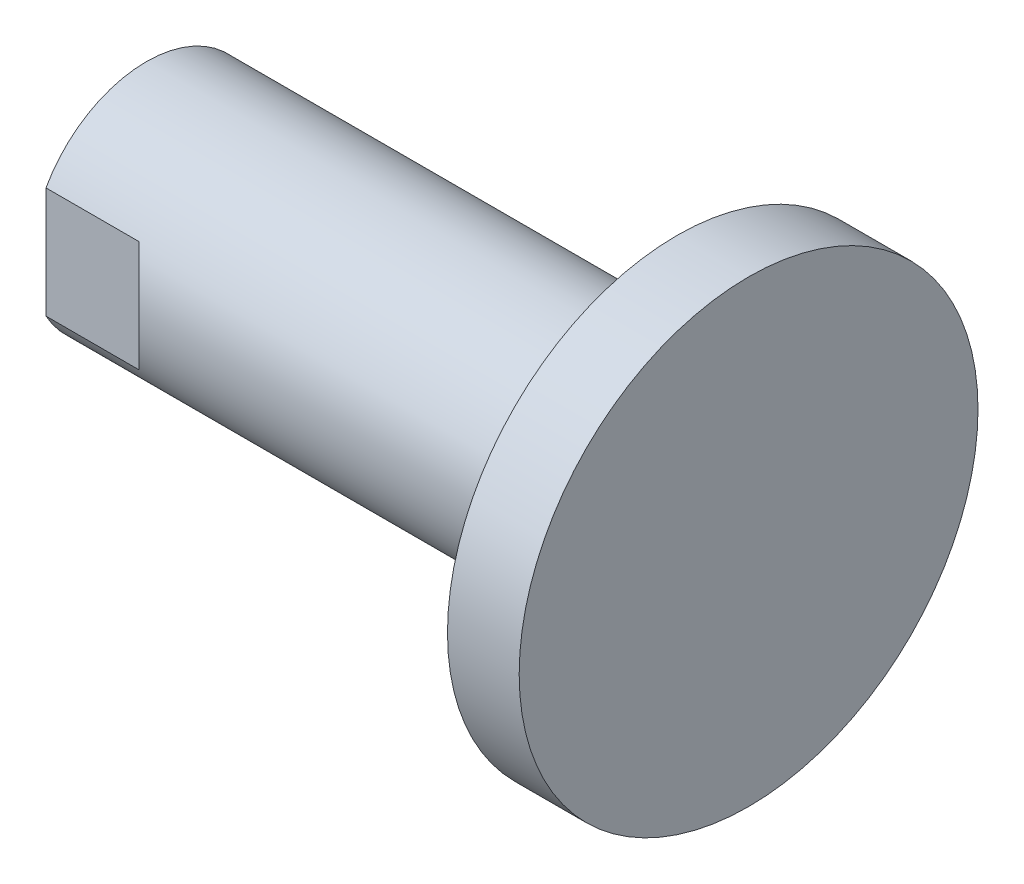
from build123d import *

# Parameters (mm, degrees)
CUT_EXTRUDE1_DEPTH      = 16
CUT_EXTRUDE1_DEPTH_BACK = 16


with BuildPart() as part:
    # Sketch1 → Revolve1 (revolve)
    with BuildSketch(Plane.XY, mode=Mode.PRIVATE) as revolve1_sk:
        Polygon((7.91882362, 0), (6, 3.3235), (-6.3235, 3.3235), (-7, 4), (-7, 8), (30, 8), (30, 16), (35, 16), (35, 0), align=None)
    revolve(revolve1_sk.sketch.rotate(Axis((35, 0, 0), (-1, 0, 0)), 270), axis=Axis((35, 0, 0), (-1, 0, 0)))

    # Sketch2 → Cut-Extrude1 (cut, two sides: drawn at the far end of the back side and taken through both)
    with BuildSketch(Plane(origin=(0, 0, 0), x_dir=(1, 0, 0), z_dir=(0, 1, 0)).offset(-CUT_EXTRUDE1_DEPTH_BACK)):
        Polygon((-12, 12), (-12, -12), (4.5, -12), (-0.5, -7), (-7, -7), (-7, 7), (-0.5, 7), (4.5, 12), align=None)
    extrude(amount=CUT_EXTRUDE1_DEPTH + CUT_EXTRUDE1_DEPTH_BACK, mode=Mode.SUBTRACT)


solid = part.part
